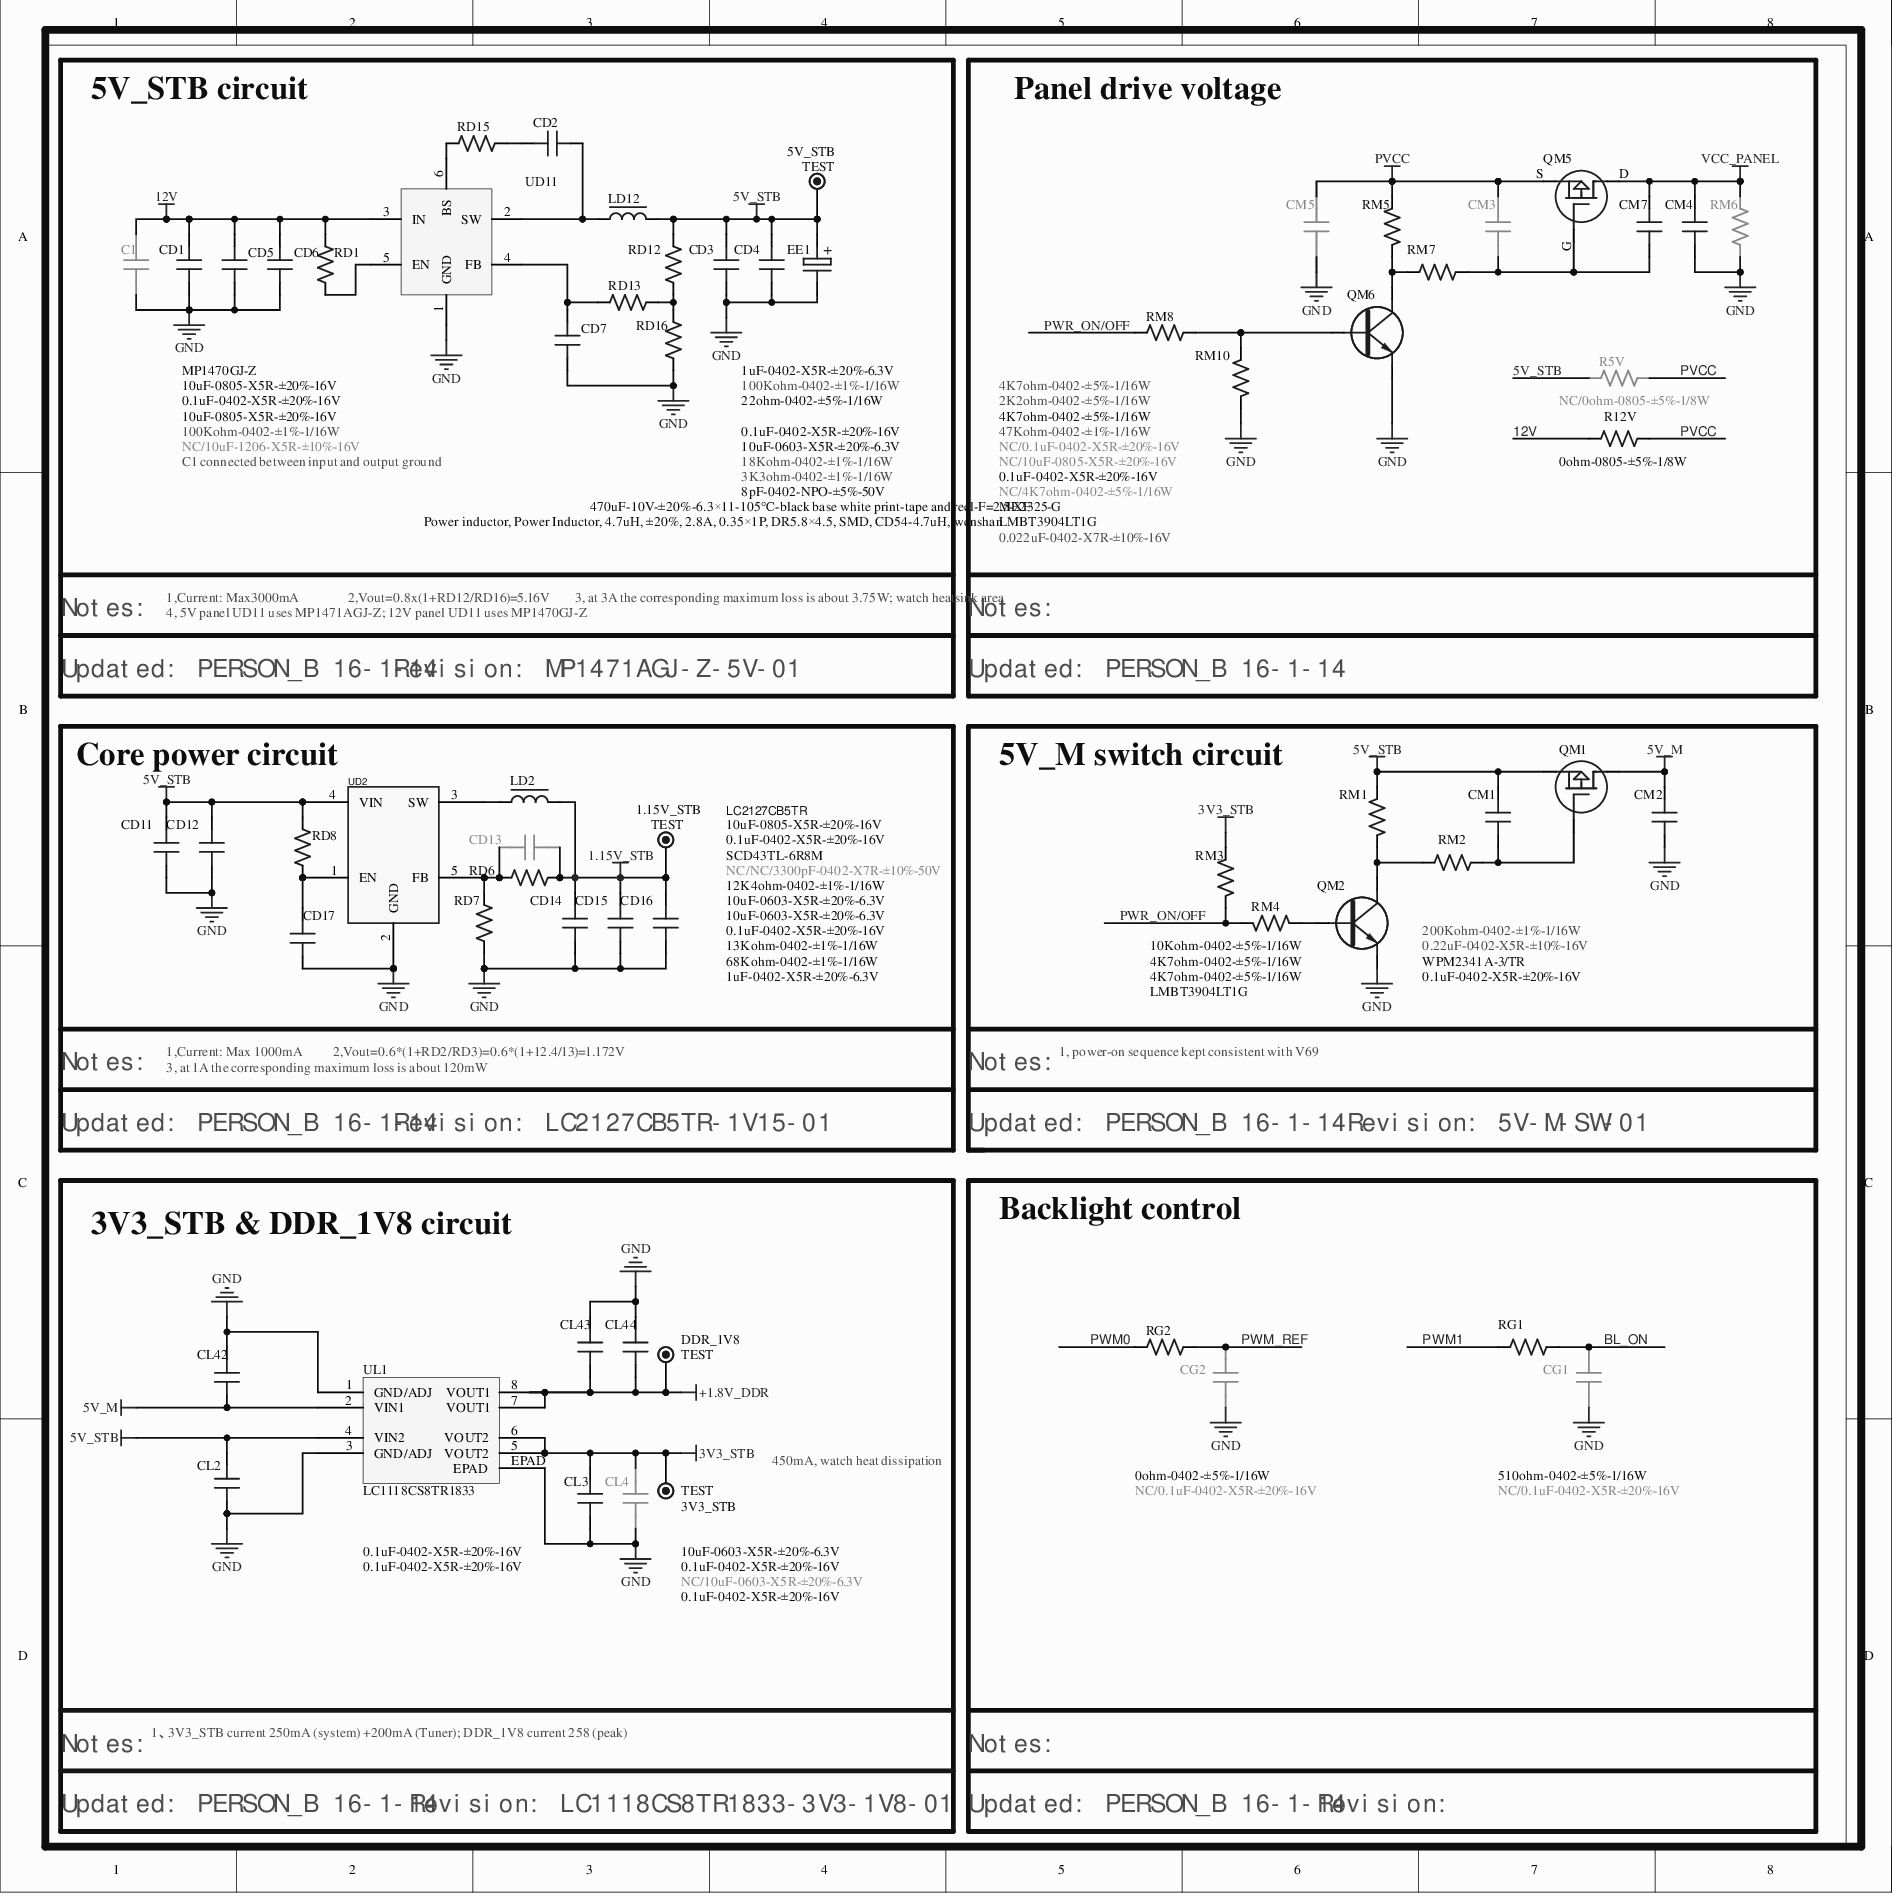
[diagram p0: MISC84277-7.SchDoc]
# Altium project MISC84277-14.PrjPCB (part 3 of 10)

## Sheet MISC84277-7.SchDoc
size 317 x 317 mm

### Parts
1.15V_STB  TEST  [TP]
3V3_STB  TEST  [TP]
5V_STB  TEST  [TP]
C1  NC/10uF-1206-X5R-±10%-16V  [C1206]
CD1  10uF-0805-X5R-±20%-16V  [C0805]
CD2  1uF-0402-X5R-±20%-6.3V  [C0402]
CD3  0.1uF-0402-X5R-±20%-16V  [C0402]
CD4  10uF-0603-X5R-±20%-6.3V  [C0603]
CD5  10uF-0805-X5R-±20%-16V  [C0805]
CD6  0.1uF-0402-X5R-±20%-16V  [C0402]
CD7  8pF-0402-NPO-±5%-50V  [C0402]
CD11  10uF-0805-X5R-±20%-16V  [C0805]
CD12  0.1uF-0402-X5R-±20%-16V  [C0402]
CD13  NC/NC/3300pF-0402-X7R-±10%-50V  [C0402]
CD14  10uF-0603-X5R-±20%-6.3V  [C0603]
CD15  10uF-0603-X5R-±20%-6.3V  [C0603]
CD16  0.1uF-0402-X5R-±20%-16V  [C0402]
CD17  1uF-0402-X5R-±20%-6.3V  [C0402]
CG1  NC/0.1uF-0402-X5R-±20%-16V  [C0402]
CG2  NC/0.1uF-0402-X5R-±20%-16V  [C0402]
CL2  0.1uF-0402-X5R-±20%-16V  [C0402]
CL3  0.1uF-0402-X5R-±20%-16V  [C0402]
CL4  NC/10uF-0603-X5R-±20%-6.3V  [C0603]
CL42  0.1uF-0402-X5R-±20%-16V  [C0402]
CL43  0.1uF-0402-X5R-±20%-16V  [C0402]
CL44  10uF-0603-X5R-±20%-6.3V  [C0603]
CM1  0.22uF-0402-X5R-±10%-16V  [C0402]
CM2  0.1uF-0402-X5R-±20%-16V  [C0402]
CM3  NC/0.1uF-0402-X5R-±20%-16V  [C0402]
CM4  0.1uF-0402-X5R-±20%-16V  [C0402]
CM5  NC/10uF-0805-X5R-±20%-16V  [C0805]
CM7  0.022uF-0402-X7R-±10%-16V  [C0402]
DDR_1V8  TEST  [TP]
EE1  470uF-10V-±20%-6.3×11-105℃-black base white print-tape and reel-F=2.5-XF  [EC(6.3*11)-V-2.5]
LD2  SCD43TL-6R8M  [L(4.5*3.5)-S]
LD12  Power inductor, Power Inductor, 4.7uH, ±20%, 2.8A, 0.35×1P, DR5.8×4.5, SMD, CD54-4.7uH, wenshan  [L(5.8*4.5)-S]
QM1  WPM2341A-3/TR  [SOT-23-1]
QM2  LMBT3904LT1G  [SOT-23]
QM5  ME2325-G  [SOT-23-1]
QM6  LMBT3904LT1G  [SOT-23]
R5V  NC/0ohm-0805-±5%-1/8W  [R0805]
R12V  0ohm-0805-±5%-1/8W  [R0805]
RD1  100Kohm-0402-±1%-1/16W  [R0402]
RD6  12K4ohm-0402-±1%-1/16W  [R0402]
RD7  13Kohm-0402-±1%-1/16W  [R0402]
RD8  68Kohm-0402-±1%-1/16W  [R0402]
RD12  18Kohm-0402-±1%-1/16W  [R0402]
RD13  100Kohm-0402-±1%-1/16W  [R0402]
RD15  22ohm-0402-±5%-1/16W  [R0402]
RD16  3K3ohm-0402-±1%-1/16W  [R0402]
RG1  510ohm-0402-±5%-1/16W  [R0402]
RG2  0ohm-0402-±5%-1/16W  [R0402]
RM1  4K7ohm-0402-±5%-1/16W  [R0402]
RM2  200Kohm-0402-±1%-1/16W  [R0402]
RM3  10Kohm-0402-±5%-1/16W  [R0402]
RM4  4K7ohm-0402-±5%-1/16W  [R0402]
RM5  4K7ohm-0402-±5%-1/16W  [R0402]
RM6  NC/4K7ohm-0402-±5%-1/16W  [R0402]
RM7  47Kohm-0402-±1%-1/16W  [R0402]
RM8  4K7ohm-0402-±5%-1/16W  [R0402]
RM10  2K2ohm-0402-±5%-1/16W  [R0402]
UD2  LC2127CB5TR  [SOT-23-5]
UD11  MP1470GJ-Z  [SOT-23-6]
UL1  LC1118CS8TR1833  [SOP8/1.27-3]

### Blocks framed on the sheet
5V_STB circuit: 5V_STB C1 CD1-CD7 EE1 LD12 RD1 RD12 RD13 RD15 RD16 UD11
Panel drive voltage: CM3-CM5 CM7 QM5 QM6 R5V R12V RM5-RM8 RM10
Core power circuit: 1.15V_STB CD11-CD17 LD2 RD6-RD8 UD2
3V3_STB & DDR_1V8 circuit: 3V3_STB CL2-CL4 CL42-CL44 DDR_1V8 UL1
Backlight control: CG1 CG2 RG1 RG2

### Nets
1.15V_STB: 1.15V_STB.1 CD13.1 CD14.2 CD15.2 CD16.2 LD2.2 RD6.2
3V3_STB: 3V3_STB.1 CL3.1 CL4.1 RM3.1 UL1.5(VOUT2) UL1.6(VOUT2)
5V_M: CL42.1 CM2.1 QM1.D UL1.2(VIN1)
5V_STB: 5V_STB.1 CD3.1 CD4.2 CD11.2 CD12.1 CL2.2 CM1.1 EE1.1 LD12.2 QM1.S R5V.1 RD8.1 RD12.2 RM1.2 UD2.4(VIN) UL1.4(VIN2)
12V: C1.2 CD1.1 CD5.1 CD6.1 R12V.1 RD1.1 UD11.3(IN)
+1.8V_DDR: CL43.2 CL44.1 DDR_1V8.1 UL1.7(VOUT1) UL1.8(VOUT1)
BL_ON: CG1.1 RG1.1
GND: C1.1 CD1.2 CD3.2 CD4.1 CD5.2 CD6.2 CD7.2 CD11.1 CD12.2 CD14.1 CD15.1 CD16.1 CD17.1 CG1.2 CG2.2 CL2.1 CL3.2 CL4.2 CL42.2 CL43.1 CL44.2 CM2.2 CM4.2 CM5.1 EE1.2 QM2.E QM6.E RD7.1 RD16.1 RM6.2 RM10.2 UD2.2(GND) UD11.1(GND) UL1.1(GND/ADJ) UL1.3(GND/ADJ) UL1.EPAD
PVCC: CM3.2 CM5.2 QM5.S R5V.2 R12V.2 RM5.2
PWM_REF: CG2.1 RG2.2
VCC_PANEL: CM4.1 CM7.1 QM5.D RM6.1
PWM0: RG2.1
PWM1: RG1.2
PWR_ON/OFF: RM3.2 RM4.2 RM8.1
NetCD2_1: CD2.1 LD12.1 UD11.2(SW)
NetCD2_2: CD2.2 RD15.2
NetCD7_1: CD7.1 RD13.2 UD11.4(FB)
NetCD13_2: CD13.2 RD6.1 RD7.2 UD2.5(FB)
NetCD17_2: CD17.2 RD8.2 UD2.1(EN)
NetCM1_2: CM1.2 QM1.G RM2.2
NetCM3_1: CM3.1 CM7.2 QM5.G RM7.2
NetLD2_1: LD2.1 UD2.3(SW)
NetQM2_B: QM2.B RM4.1
NetQM2_C: QM2.C RM1.1 RM2.1
NetQM6_B: QM6.B RM8.2 RM10.1
NetQM6_C: QM6.C RM5.1 RM7.1
NetRD1_2: RD1.2 UD11.5(EN)
NetRD12_1: RD12.1 RD13.1 RD16.2
NetRD15_1: RD15.1 UD11.6(BS)

### Notes on the sheet
- C1 connected between input and output ground
- Notes:
- 1,Current: Max3000mA
- 4, 5V panel UD11 uses MP1471AGJ-Z; 12V panel UD11 uses MP1470GJ-Z
- 2,Vout=0.8x(1+RD12/RD16)=5.16V
- 3, at 3A the corresponding maximum loss is about 3.75W; watch heatsink area
- Updated: PERSON_B 16-1-14
- Revision: MP1471AGJ-Z-5V-01
- 5V_M switch circuit
- 1,Current: Max 1000mA
- 3, at 1A the corresponding maximum loss is about 120mW
- 2,Vout=0.6*(1+RD2/RD3)=0.6*(1+12.4/13)=1.172V
- 1, power-on sequence kept consistent with V69
- Revision: LC2127CB5TR-1V15-01
- Revision: 5V-M-SW-01
- 450mA, watch heat dissipation
- 1、3V3_STB current 250mA (system) +200mA (Tuner); DDR_1V8 current 258 (peak)
- Revision: LC1118CS8TR1833-3V3-1V8-01
- Revision:

### Library data of the parts
C1 = 10uF-1206-X5R-±10%-16V-D
CD1 CD5 CM5 = 10uF-0805-X5R-±20%-16V-D
CD2 CD3 CD6 CL2 CL3 CL42 CL43 = 0.1uF-0402-X5R-±20%-16V-D
CD4 CD11 CD14 CD15 CL4 CL44 = 10uF-0603-X5R-±20%-6.3V-D
CD7 = 10pF-0402-NPO-±5%-50V-D
CD12 CD16 CD17 CG1 CG2 CM1 CM2 CM4 = 0.1uF-0402-Y5V-+80%-20%-16V-D
CD13 = 3300pF-0402-X7R-±10%-50V-D
CM3 = 0.22uF-0402-Y5V-+80%-20%-16V-D
CM7 = 0.01uF-0402-X7R-±10%-50V-D
EE1 = 470uF-10V-±20%-6.3×11-105℃-黑底白字-编带-F=2.5-XF-DHAI: Electrolytic
LD2 = CTD0403-6R8-M-D
LD12 = CTD0504-4R7-M-D: Text Field1: 20; Text Field2: 40
QM1 = WPM2341A-3/TR-D
QM2 QM6 = LMBT3904LT1G-D-NPN: Q-NPN-#-#-#
QM5 = WPM3407C-3/TR-D
R5V R12V = 0ohm-0805-±5%-1/8W-D
RD1 RM2 = 100Kohm-0402-±5%-1/16W-D
RD6 = 12Kohm-0402-±1%-1/16W-D
RD7 = 12K4ohm-0402-±1%-1/16W-D
RD8 = 47Kohm-0402-±5%-1/16W-D
RD12 = 30Kohm-0402-±1%-1/16W-D
RD13 RG2 = 0ohm-0402-±5%-1/16W-D
RD15 = 22ohm-0402-±5%-1/16W-D
RD16 = 5K6ohm-0402-±1%-1/16W-D
RG1 = 510ohm-0402-±5%-1/16W-D
RM1 RM5 RM6 = 4k7ohm-0402-±5%-1/16W-D
RM3 RM4 = 10Kohm-0402-±5%-1/16W-D
RM7 = 200Kohm-0402-±5%-1/16W-D
RM8 = 100ohm-0402-±5%-1/16W-D
RM10 = 2K2ohm-0402-±5%-1/16W-D
UD2 = LC3406CB5TR-D
UD11 = RT6212
UL1 = LC1118-D